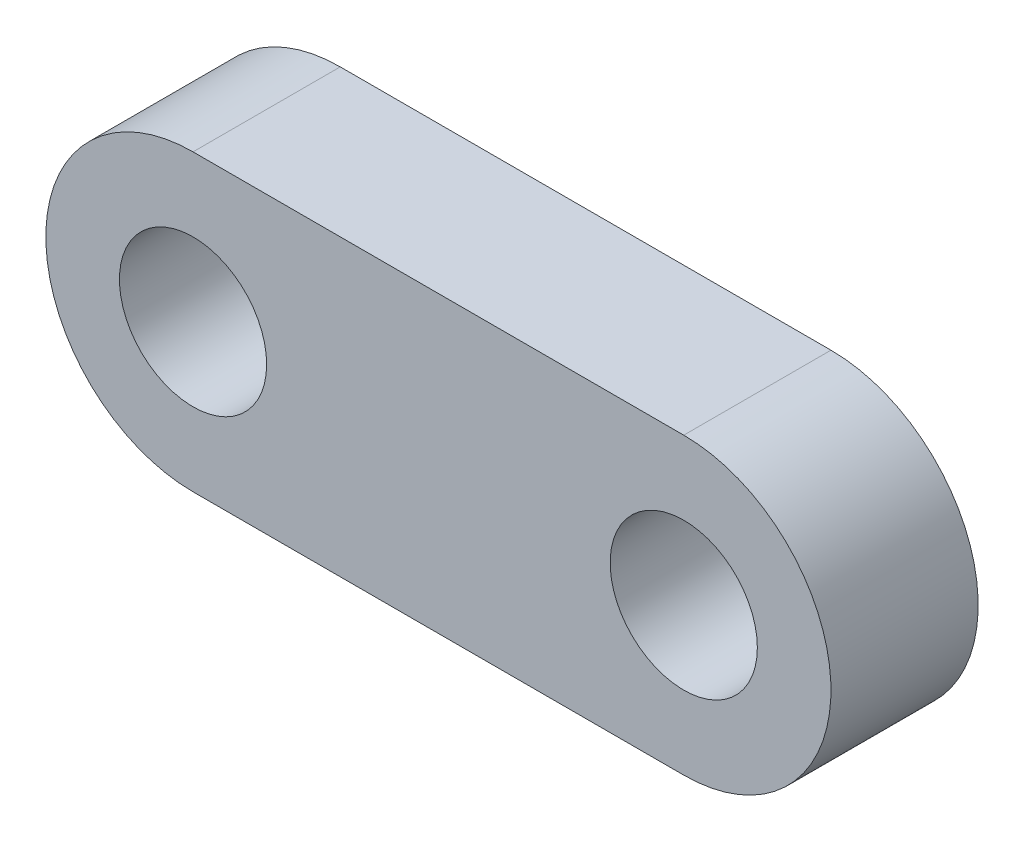
from build123d import *

# Parameters (mm, degrees)
SKETCH1_R           = 1.5
BOSS_EXTRUDE1_DEPTH = 3


with BuildPart() as part:
    # Sketch1 → Boss-Extrude1 (new body)
    with BuildSketch(Plane.XY):
        with BuildLine():
            Line((0, 3), (10, 3))
            ThreePointArc((10, 3), (13, 0), (10, -3))
            Line((10, -3), (0, -3))
            ThreePointArc((0, -3), (-3, 0), (0, 3))
        make_face()
        Circle(SKETCH1_R, mode=Mode.SUBTRACT)
        with Locations((10, 0)):
            Circle(SKETCH1_R, mode=Mode.SUBTRACT)
    extrude(amount=BOSS_EXTRUDE1_DEPTH)


solid = part.part
